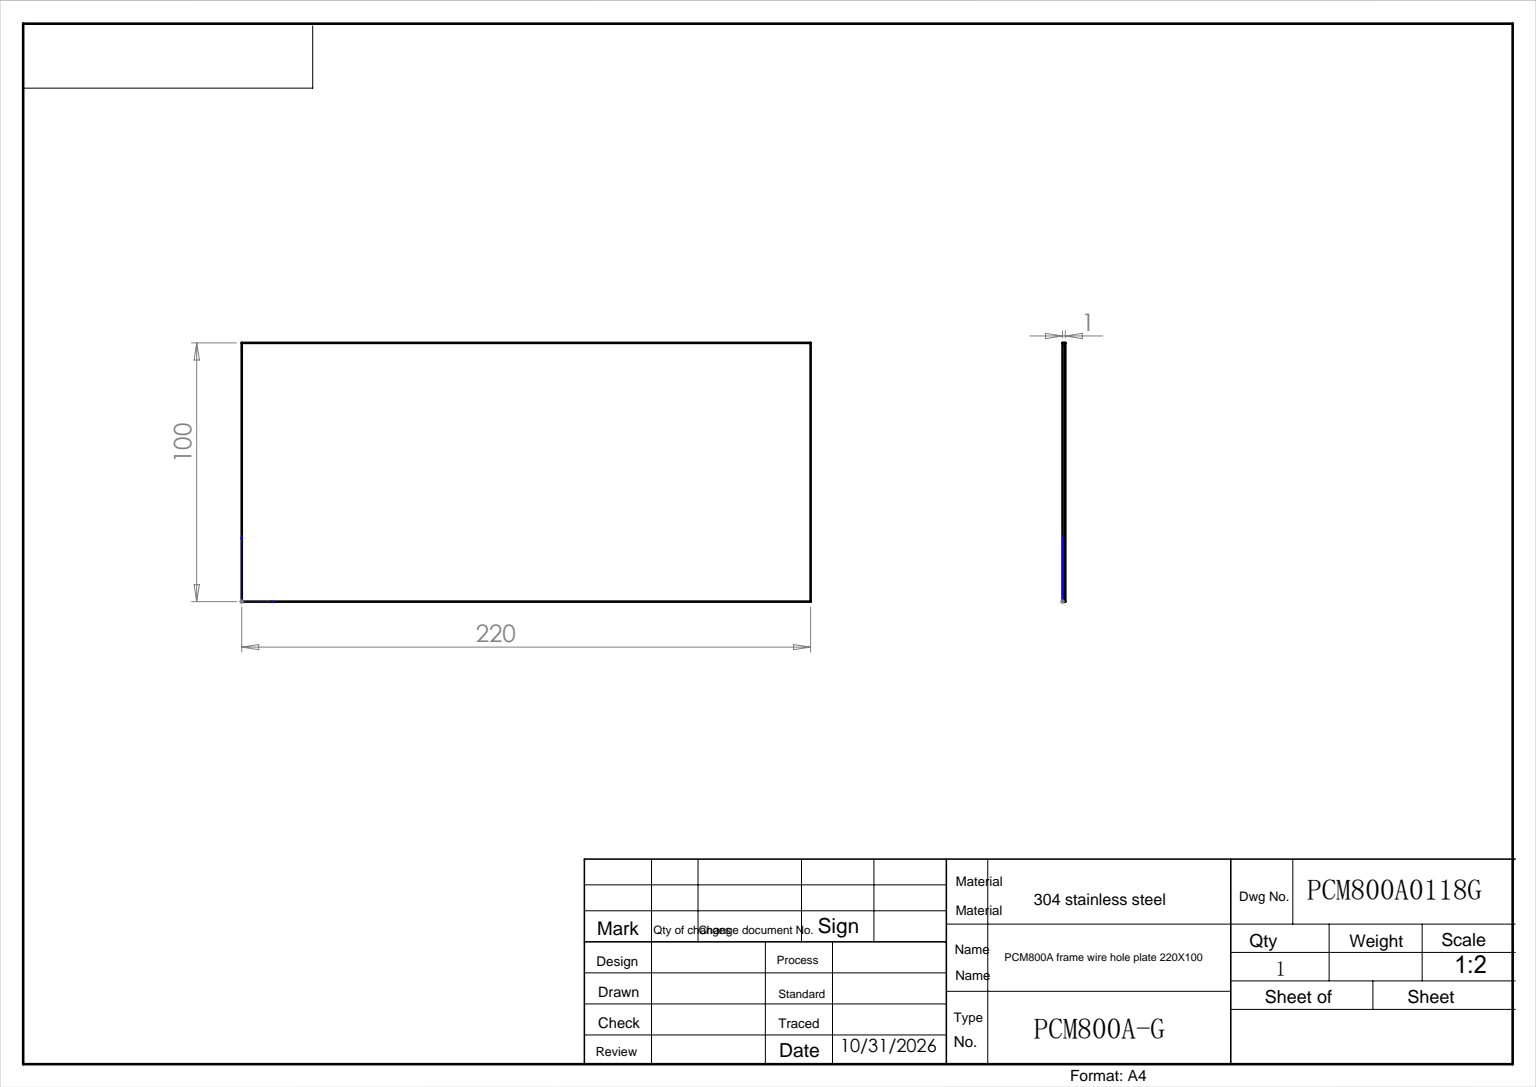
from build123d import *

# Parameters (mm, degrees)
SKETCH_1_W      = 220
SKETCH_1_H      = 100
EXTRUDE_1_DEPTH = 1


with BuildPart() as part:
    # 草图1 → 凸台-拉伸1 (new body)
    with BuildSketch(Plane.XY):
        with Locations((110, 50)):
            Rectangle(SKETCH_1_W, SKETCH_1_H)
    extrude(amount=EXTRUDE_1_DEPTH)


solid = part.part
